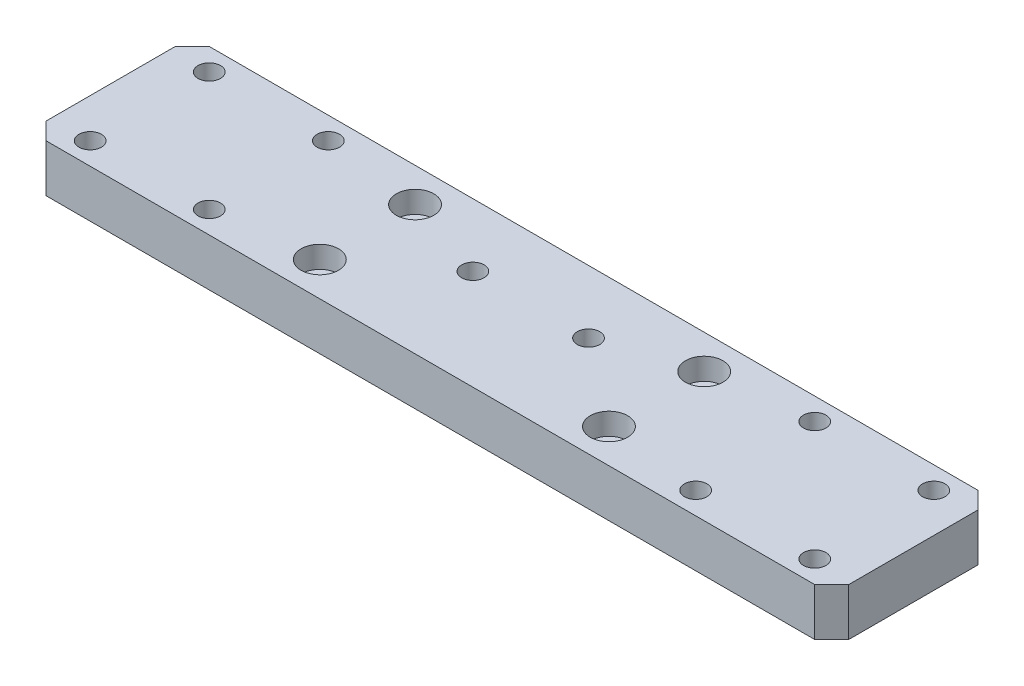
from build123d import *

# Parameters (mm, degrees)
SKETCH_2_W                   = 236
SKETCH_2_H                   = 14
EXTRUDE_1_DEPTH              = 48
HOLE_WIZARD_M6_1_D           = 6.6
HOLE_WIZARD_M6_1_DEPTH       = 14
HOLE_WIZARD_M6_1_CBORE_D     = 11
HOLE_WIZARD_M6_1_CBORE_DEPTH = 6.4
HOLE_WIZARD_M6_1_TIP         = 1.982840043
CHAMFER_1_SIZE               = 5
HOLE_WIZARD_M6_2_D           = 6.6
HOLE_WIZARD_M6_2_DEPTH       = 14
HOLE_WIZARD_M6_2_CBORE_D     = 11
HOLE_WIZARD_M6_2_CBORE_DEPTH = 6.4
HOLE_WIZARD_M6_2_TIP         = 1.982840043
HOLE_WIZARD_M6_1_2_D         = 6.6


with BuildPart() as part:
    # 草图2 → 凸台-拉伸1 (new body)
    with BuildSketch(Plane.XY):
        with Locations((118, -7)):
            Rectangle(SKETCH_2_W, SKETCH_2_H)
    extrude(amount=EXTRUDE_1_DEPTH)

    # Hole Wizard M6 _1
    with Locations(Plane(origin=(0, -14, 0), x_dir=(-1, 0, 0), z_dir=(0, -1, 0))):
        with Locations((-224.5, -6.5), (-189.5, -6.5), (-189.5, -41.5), (-224.5, -41.5), (-11.5, -41.5), (-46.5, -41.5), (-46.5, -6.5), (-11.5, -6.5)):
            CounterBoreHole(HOLE_WIZARD_M6_1_D / 2, HOLE_WIZARD_M6_1_CBORE_D / 2, HOLE_WIZARD_M6_1_CBORE_DEPTH, depth=HOLE_WIZARD_M6_1_DEPTH)
            with Locations((0, 0, -(HOLE_WIZARD_M6_1_DEPTH + HOLE_WIZARD_M6_1_TIP / 2))):  # 118° drill point
                Cone(0, HOLE_WIZARD_M6_1_D / 2, HOLE_WIZARD_M6_1_TIP, mode=Mode.SUBTRACT)

    # 倒角1
    chamfer_1_edges = [part.edges().sort_by_distance(p)[0] for p in [
        (236, -7, 48),
        (0, -7, 48),
        (236, -7, 0),
        (0, -7, 0),
    ]]
    chamfer(chamfer_1_edges, length=CHAMFER_1_SIZE)

    # M6 六角凹头螺钉的柱形沉头孔2
    with Locations(Plane(origin=(0, 0, 0), x_dir=(1, 0, 0), z_dir=(0, 1, 0))):
        with Locations((75.5, -10), (160.5, -10), (75.5, -38), (160.5, -38)):
            CounterBoreHole(HOLE_WIZARD_M6_2_D / 2, HOLE_WIZARD_M6_2_CBORE_D / 2, HOLE_WIZARD_M6_2_CBORE_DEPTH, depth=HOLE_WIZARD_M6_2_DEPTH)
            with Locations((0, 0, -(HOLE_WIZARD_M6_2_DEPTH + HOLE_WIZARD_M6_2_TIP / 2))):  # 118° drill point
                Cone(0, HOLE_WIZARD_M6_2_D / 2, HOLE_WIZARD_M6_2_TIP, mode=Mode.SUBTRACT)

    # Hole Wizard M6 _1 2 (through all)
    with Locations(Plane(origin=(0, 0, 0), x_dir=(1, 0, 0), z_dir=(0, 1, 0))):
        with Locations((101, -18.5), (135, -18.5)):
            Hole(HOLE_WIZARD_M6_1_2_D / 2)


solid = part.part
